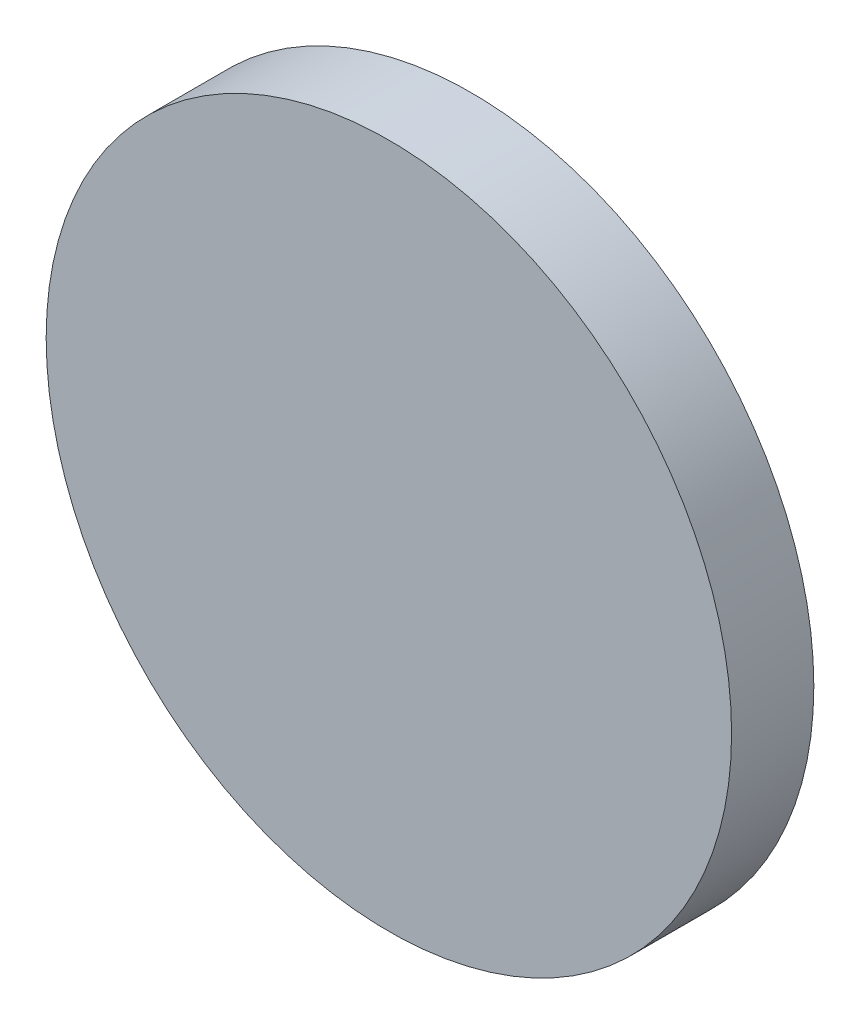
SolidWorks part; units mm, degrees
material "Q235-A"
ref_plane "前视基准面" through (0, 0, 0) normal (0, 0, 1) x (1, 0, 0)
ref_plane "上视基准面" through (0, 0, 0) normal (0, 1, 0) x (1, 0, 0)
ref_plane "右视基准面" through (0, 0, 0) normal (1, 0, 0) x (0, 0, -1)
sketch "草图1" plane through (0, 0, 0) normal (0, 0, 1) x (1, 0, 0)
  circle A0 centre (0, 0) radius 25
  dimension "D1" = 50
extrude "凸台-拉伸1" add sketch "草图1" along normal blind 6
